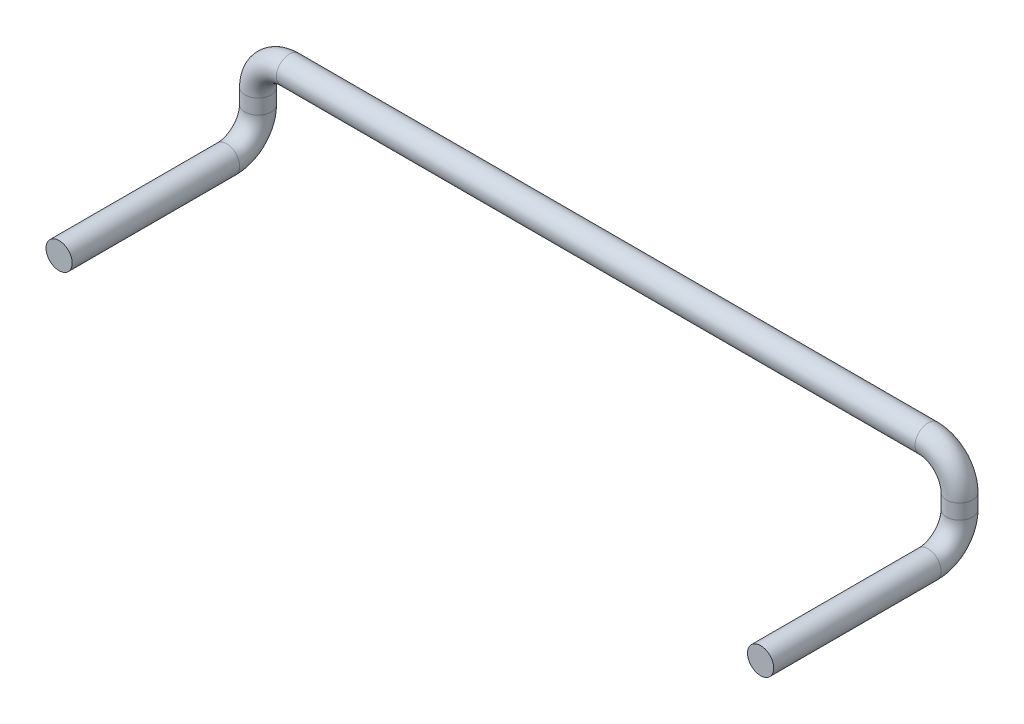
from build123d import *

# Parameters (mm, degrees)
SWEEP1_PROFILE_R = 12.5


with BuildPart() as part:
    # Sweep1: sweep along a curve in space
    with BuildLine() as sweep1_path:
        Line((335, -74.161984871, 30), (335, -74.161984871, 190))
        ThreePointArc((335, -74.161984871, 30), (335, -65.375188307, 8.786796564), (335, -44.161984871, 0))
        Line((335, -30, 0), (335, -44.161984871, 0))
        ThreePointArc((335, -30, 0), (326.213203436, -8.786796564, 0), (305, 0, 0))
        Line((-305, 0, 0), (305, 0, 0))
        ThreePointArc((-305, 0, 0), (-326.213203436, -8.786796564, 0), (-335, -30, 0))
        Line((-335, -30, 0), (-335, -44.161984871, 0))
        ThreePointArc((-335, -74.161984871, 30), (-335, -65.375188307, 8.786796564), (-335, -44.161984871, 0))
        Line((-335, -74.161984871, 30), (-335, -74.161984871, 190))
    # Sweep1 profile (on start of the path) → Sweep1 (sweep)
    with BuildSketch(Plane(origin=(-335, -74.161984871, 190), x_dir=(-1, 0, 0), z_dir=(0, 0, -1))):
        Circle(SWEEP1_PROFILE_R)
    sweep(path=sweep1_path.line)


solid = part.part
